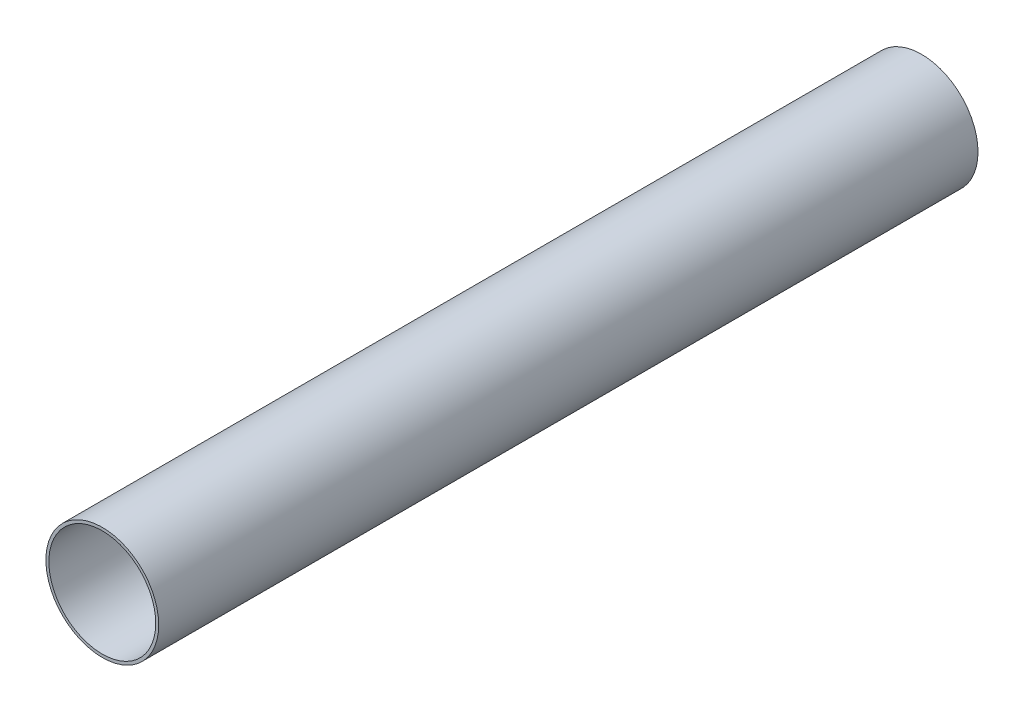
from build123d import *

# Parameters (mm, degrees)
SKETCH_1_R      = 47.5
SKETCH_1_R_2    = 45
EXTRUDE_1_DEPTH = 345


with BuildPart() as part:
    # 草图1 → 凸台-拉伸1 (new, symmetric)
    with BuildSketch(Plane.XY):
        Circle(SKETCH_1_R)
        Circle(SKETCH_1_R_2, mode=Mode.SUBTRACT)
    extrude(amount=EXTRUDE_1_DEPTH, both=True)


solid = part.part
